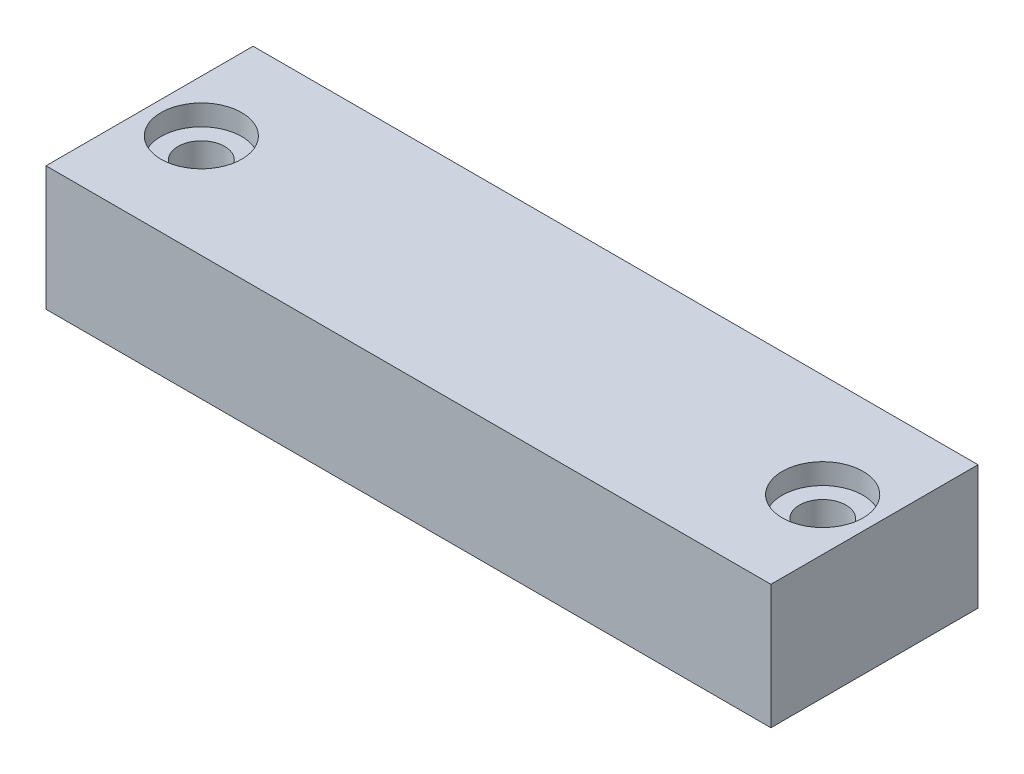
SolidWorks part; units mm, degrees
material "黄铜"
ref_plane "前视基准面" through (0, 0, 0) normal (0, 0, 1) x (1, 0, 0)
ref_plane "上视基准面" through (0, 0, 0) normal (0, 1, 0) x (1, 0, 0)
ref_plane "右视基准面" through (0, 0, 0) normal (1, 0, 0) x (0, 0, -1)
sketch "草图1" plane through (0, 0, 0) normal (0, 1, 0) x (1, 0, 0)
  line L1 (-35, 10) -> (35, 10)
  line L2 (-35, 10) -> (-35, -10)
  line L3 (-35, -10) -> (35, -10)
  line L4 (35, 10) -> (35, -10)
  line L5 (-35, 10) -> (35, -10) construction
  line L6 (-35, -10) -> (35, 10) construction
  point P0 (0, 0)
  dimension "D1" = 20
  dimension "D2" = 70
extrude "凸台-拉伸1" add sketch "草图1" along normal blind 12
hole_wizard "打孔尺寸(%根据)内六角圆柱头螺钉的类型1" positions "草图3" profile "草图2" counterbore size "M4" standard "GB" end condition through all
sketch "草图3" plane through (0, 12, 0) normal (0, 1, 0) x (1, 0, 0)
  line L0 (0, 10) -> (0, -10) construction
  line L1 (35, 10) -> (-35, 10) construction
  line L2 (-35, -10) -> (35, -10) construction
  point P0 (-30, 0)
  point P13 (30, 0)
  dimension "D1" = 60
sketch "草图2" plane through (-30, 12, 0) normal (1, 0, 0) x (0, 0, 1)
  line L0 (0, 0) -> (0, 12)
  line L1 (0, 12) -> (2.25, 12)
  line L3 (2.25, 12) -> (2.25, 2)
  line L4 (2.25, 2) -> (3.9, 2)
  line L5 (3.9, 2) -> (3.9, 0)
  line L7 (3.9, 0) -> (0, 0)
  line L11 (0, -6.35) -> (0, 107.95) construction
  dimension "通孔孔直径" = 4.5
  dimension "通孔孔深度" = 12
  dimension "柱形沉头孔直径" = 7.8
  dimension "柱形沉头孔深度" = 2
